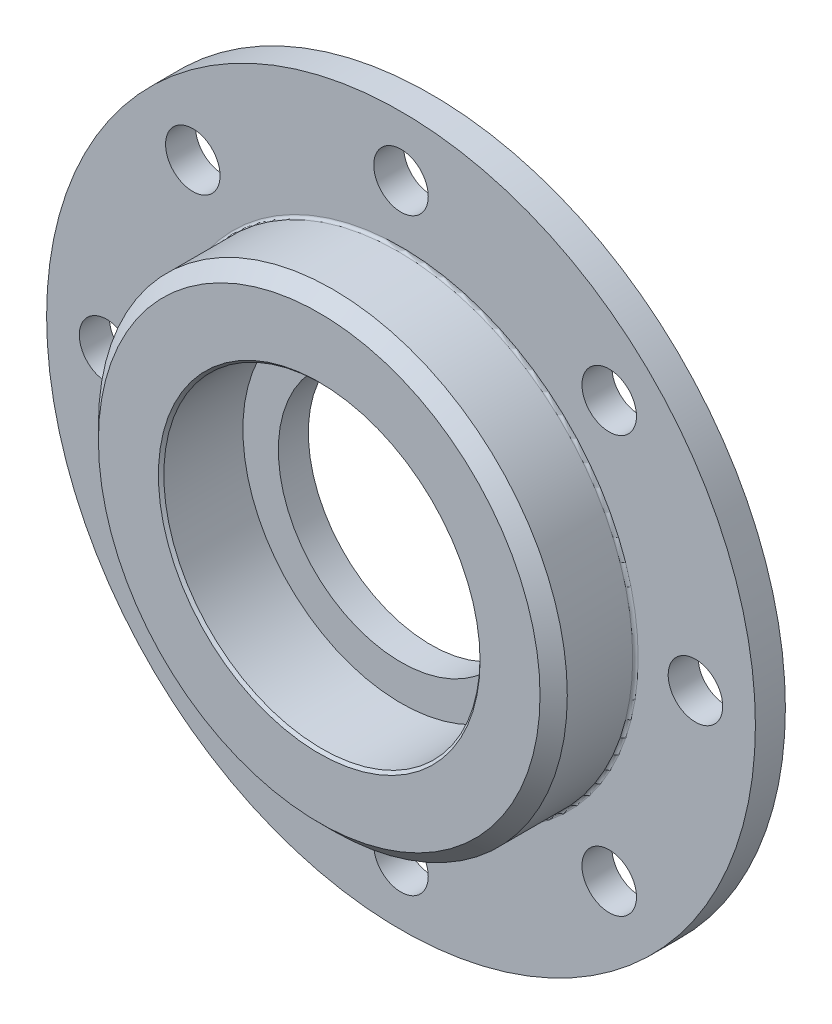
from build123d import *

# Parameters (mm, degrees)
SKETCH_1_R               = 130
EXTRUDE_1_DEPTH          = 11
SKETCH_2_R               = 86
SKETCH_2_R_2             = 58
EXTRUDE_2_DEPTH          = 30
FILLET_1_R               = 1
CHAMFER_1_SIZE           = 1
CHAMFER_2_SIZE           = 5
CUT_EXTRUDE_1_REACH      = 190.364
SKETCH_4_R               = 10
PATTERN_CIRCULAR_1_COUNT = 8
SKETCH_5_R               = 45
CUT_EXTRUDE_2_DEPTH      = 187.279360102


with BuildPart() as part:
    # 草图1 → 凸台-拉伸1 (new body)
    with BuildSketch(Plane.XY):
        Circle(SKETCH_1_R)
    extrude(amount=EXTRUDE_1_DEPTH)

    # 草图2 → 凸台-拉伸2 (add)
    with BuildSketch(Plane.XY.offset(11)):
        Circle(SKETCH_2_R)
        Circle(SKETCH_2_R_2, mode=Mode.SUBTRACT)
    extrude(amount=EXTRUDE_2_DEPTH)

    # 圆角1
    fillet_1_edges = [part.edges().sort_by_distance(p)[0] for p in [
        (-86, 0, 11),
    ]]
    fillet(fillet_1_edges, radius=FILLET_1_R)

    # 倒角1
    chamfer_1_edges = [part.edges().sort_by_distance(p)[0] for p in [
        (-58, 0, 41),
    ]]
    chamfer(chamfer_1_edges, length=CHAMFER_1_SIZE)

    # 倒角2
    chamfer_2_edges = [part.edges().sort_by_distance(p)[0] for p in [
        (-86, 0, 41),
    ]]
    chamfer(chamfer_2_edges, length=CHAMFER_2_SIZE)

    # 草图4 → 切除-拉伸1 (cut, up to next)
    with BuildSketch(Plane(origin=(0, 0, 0), x_dir=(-1, 0, 0), z_dir=(0, 0, -1)), mode=Mode.PRIVATE) as cut_extrude_1_sk1:
        with Locations((0, 108)):
            Circle(SKETCH_4_R)
    cut_extrude_1_tool1 = extrude(cut_extrude_1_sk1.sketch, amount=-CUT_EXTRUDE_1_REACH, mode=Mode.PRIVATE) & part.part
    cut_extrude_1 = cut_extrude_1_tool1.solids().sort_by_distance((0, 108, 0))[0]
    add(cut_extrude_1, mode=Mode.SUBTRACT)

    # 阵列(圆周)1: 切除-拉伸1 ×8 about axis
    pattern_circular_1_axis = Axis((0, 0, 0), (0, 0, 1))
    for i in range(1, PATTERN_CIRCULAR_1_COUNT):
        add(cut_extrude_1.rotate(pattern_circular_1_axis, i * 360 / PATTERN_CIRCULAR_1_COUNT), mode=Mode.SUBTRACT)

    # 草图5 → 切除-拉伸2 (cut, through all)
    with BuildSketch(Plane.XY.offset(11)):
        Circle(SKETCH_5_R)
    extrude(amount=-CUT_EXTRUDE_2_DEPTH, mode=Mode.SUBTRACT)


solid = part.part
